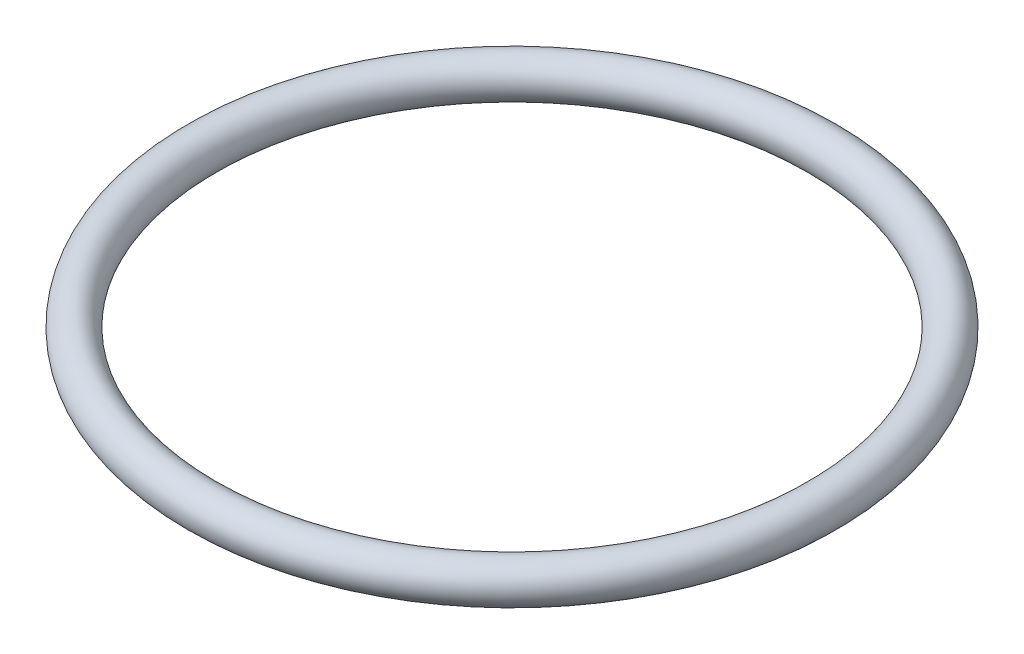
SolidWorks part; units mm, degrees
ref_plane "前视基准面" through (0, 0, 0) normal (0, 0, 1) x (1, 0, 0)
ref_plane "上视基准面" through (0, 0, 0) normal (0, 1, 0) x (1, 0, 0)
ref_plane "右视基准面" through (0, 0, 0) normal (1, 0, 0) x (0, 0, -1)
sketch "草图1" plane through (0, 0, 0) normal (0, 0, 1) x (1, 0, 0)
  line L0 (0, 0) -> (0, 14.5966) construction
  circle A0 centre (-11.75, 0) radius 0.75
  dimension "D2" = 1.5
  dimension "D1" = 23.5
revolve "旋转1" add sketch "草图1" angle 360 about L0
sketch "草图2" plane through (0, 0, 0) normal (0, 1, 0) x (1, 0, 0)
  circle A0 centre (0, 0) radius 11.7324
